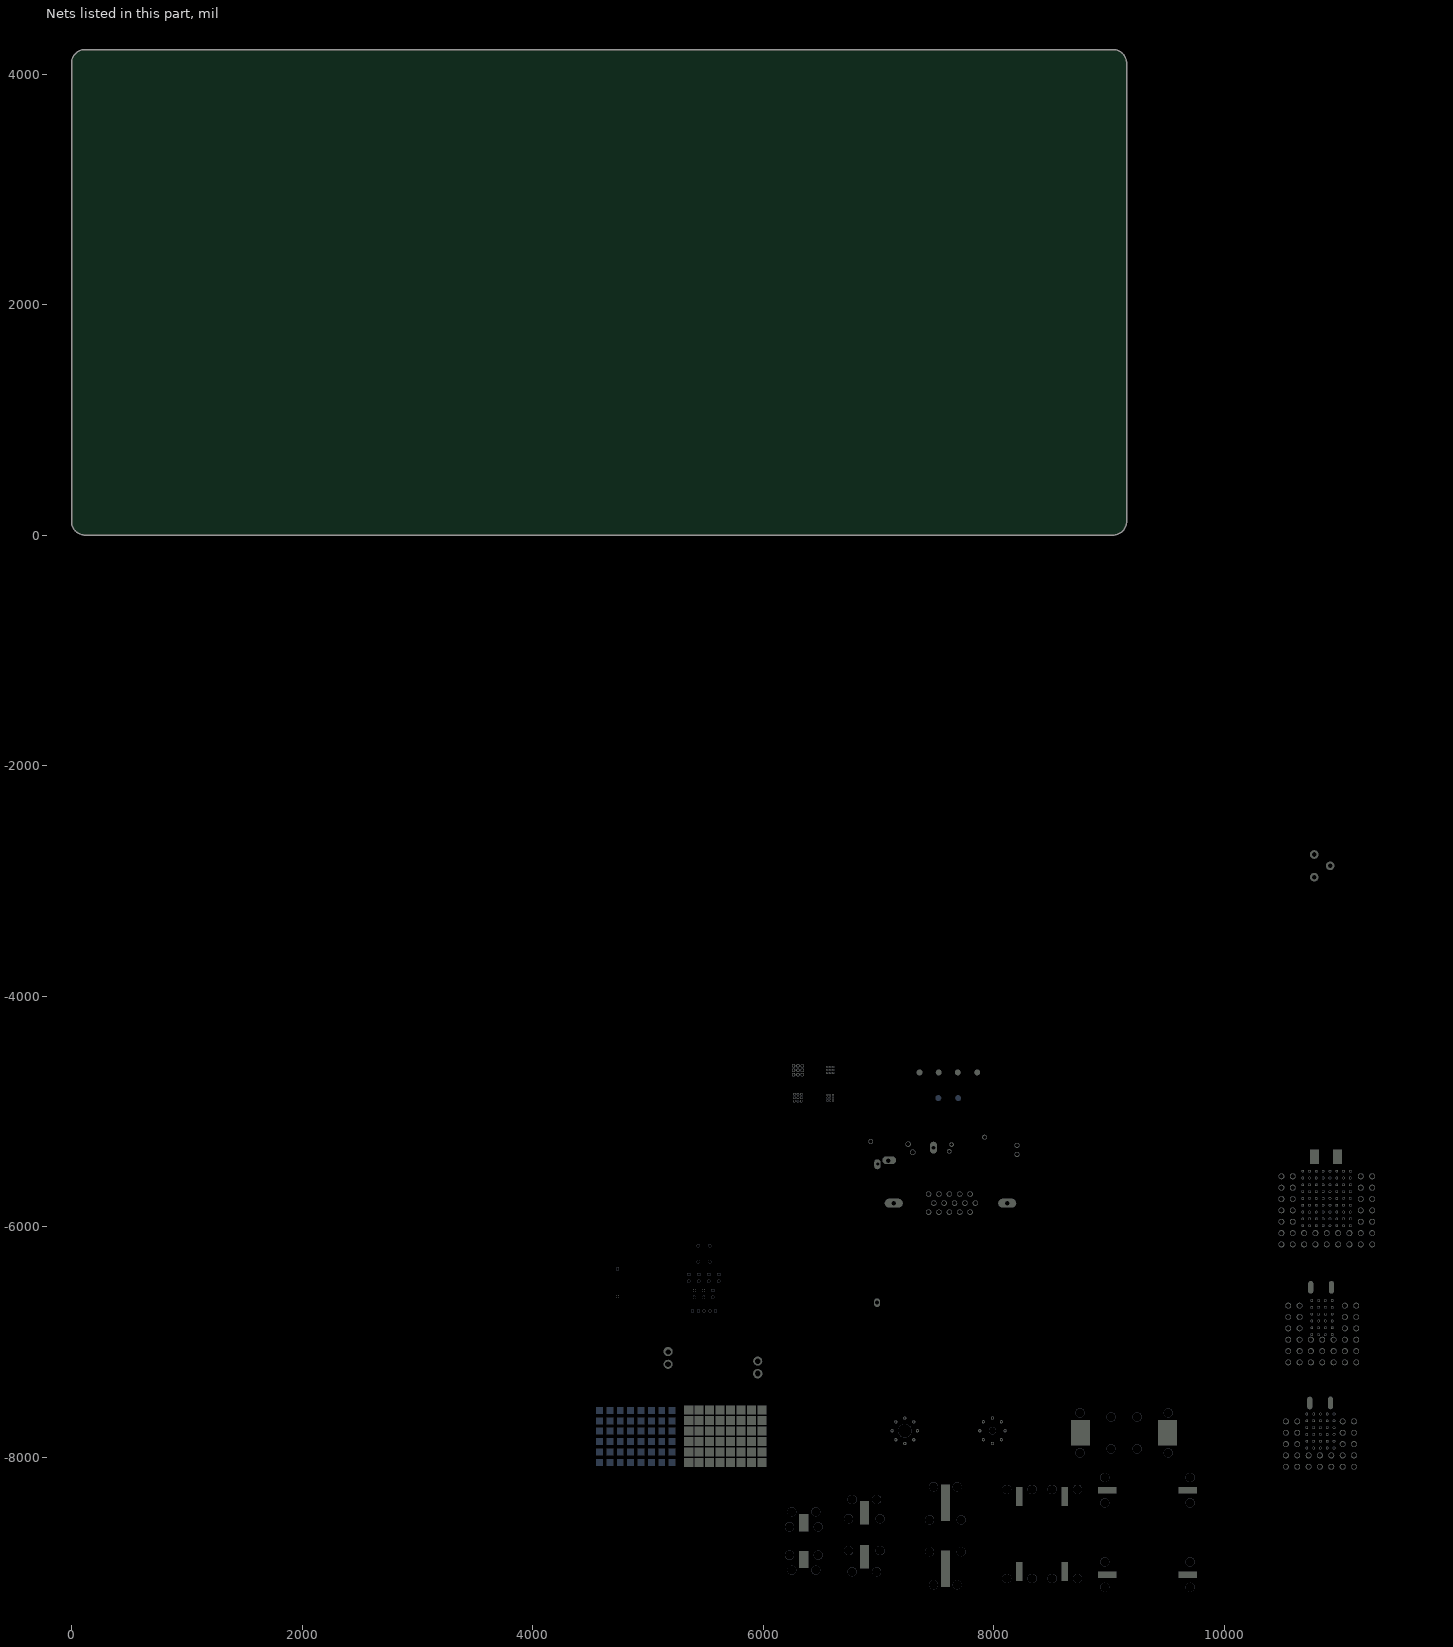
[diagram p0: the nets of this part, all layers, seen from the top]
# Altium PCB MISC86383.PcbDoc (part 2 of 2)
Units mil, origin at the board's own origin, x right, y up, seen from the top; angles counter-clockwise.
Board outline 9153.54 x 4212.6 mil, 2 copper layers (TopLayer, BottomLayer), stack 61.855 mil thick; 21 components, 2 nets, 540 pads, 0 vias.

## Nets (pads, with @x,y where several pads share a name; then routed paths per layer and width w, separated by ;. In a path a pad name is that pad's centre, name@x,y a point inside that pad or via, vN(x,y) a via of type N, cw(c..) or ccw(c..) an arc to the next point about the centre after c; other vN are vias at no path point)
GND: 
RFGND: 
pads on no net: A15XXX.0 AI_V.0 AI_V.1 AI_V.2 M1.0 M2.0 M3.0 M4.0 M5.0 M6.0 MAC.0 Manufacture_Info.0 QR1.0 QR2.0 S/N1.0 S/N2.0 XX.XXXXX.XX.0
copper on no net: | length 3400.6
  TopLayer w5: 966.99,-5983.31 966.99,-5904.57 ; 416.09,-5983.31 1148.12,-5983.31 1148.12,-5904.57 416.09,-5904.57 416.09,-5983.31
  BottomLayer w5: 966.99,-6201.16 966.99,-6122.42 ; 416.09,-6201.16 416.09,-6122.42 1148.12,-6122.42 1148.12,-6201.16 416.09,-6201.16

## Keep-outs
KeepOutLayer:
  rectangle: 416.09,-6580.59 546.29,-6501.85
  lines w5: 966.99,-6580.59 966.99,-6501.85 ; 4541.11,-6803.68 4619.85,-6803.68 ccw(c4619.85,-6685.57) 4737.96,-6685.57 4737.96,-6213.13 ; 4737.96,-6656.59 cw(c4767.4,-6686.21) 4797.02,-6656.78 4797.02,-6803.68 4836.39,-6803.68 ccw(c4836.39,-6685.57) 4954.5,-6685.57 4954.5,-6213.13 ; 4737.96,-6316.89 ccw(c4767.55,-6287.42) 4797.02,-6317.01 4797.02,-6213.13 ; 5281.04,-6265.02 5340.1,-6265.02 5340.1,-6284.67 ccw(c5359.78,-6284.67) 5359.78,-6304.36 5614.11,-6304.36 ccw(c5614.11,-6284.67) 5633.8,-6284.67 5633.8,-6264.99 5692.85,-6265.02 ; 5281.05,-6205.93 5340.1,-6205.93 5340.1,-6186.25 cw(c5359.78,-6186.25) 5359.78,-6166.56 5614.12,-6166.56 cw(c5614.12,-6186.25) 5633.8,-6186.25 5633.8,-6205.93 5692.86,-6205.93 ; 5306.95,-6473.4 ccw(c5277.42,-6443.87) 5306.95,-6414.35 ; 5338.99,-6732.15 ccw(c5309.46,-6702.63) 5338.99,-6673.1 ; 5354.45,-6611.9 ccw(c5324.92,-6582.37) 5354.45,-6552.85 ; 5407.42,-6304.36 ccw(c5338.52,-6235.46) 5407.42,-6166.56 ; 5566.48,-6304.36 cw(c5635.38,-6235.46) 5566.48,-6166.56 ; 5613.5,-6611.9 cw(c5643.03,-6582.37) 5613.5,-6552.85 ; 5637.42,-6732.15 cw(c5666.94,-6702.63) 5637.42,-6673.1 ; 5665.21,-6473.4 cw(c5694.74,-6443.87) 5665.21,-6414.35 ; 0,118.11 ccw(c118.11,118.11) 118.11,0 9035.43,0 ccw(c9035.44,118.11) 9153.55,118.11 9153.55,4094.49 ccw(c9035.44,4094.49) 9035.44,4212.6 118.11,4212.6 ccw(c118.11,4094.49) 0,4094.49 0,118.11 ; 416.09,-6580.59 416.09,-6501.85 1148.12,-6501.85 1148.12,-6580.59 416.09,-6580.59
  lines w47.24: 10850.53,-2998.7 10850.53,-2745.7
  text "KeepOutLayer" at 568.89,-6559.63 h60
  text ".GKO" at 990.7,-6562.54 h60

## Other copper
TopLayer:
  rectangle: 10382.58,-6368.37 11378.64,-5495.37
  rectangle: 10386.51,-7349.73 11311.71,-6621.38
  rectangle: 10441.74,-8196.49 11229.14,-7605.94
  rectangle: 416.09,-5983.31 546.29,-5904.57
  pour cut-out: 8822.66,-7675.58 8822.66,-7903.92 8954.55,-7903.92 8954.55,-7675.58
  pour cut-out: 9440.77,-7675.58 9440.77,-7903.92 9308.88,-7903.92 9308.88,-7675.58
  text "TopLayer" at 582.14,-5960.97 h60
  text ".GTL" at 991.63,-5965.26 h60
BottomLayer:
  rectangle: 416.09,-6201.16 546.29,-6122.42
  region: 7195.27,-5353.48 7195.53,-5353.51 7195.79,-5353.56 7196.04,-5353.62 7196.29,-5353.7 7196.54,-5353.79 7196.77,-5353.9 7197,-5354.03 7197.22,-5354.17 7197.43,-5354.32 7197.63,-5354.49 7197.82,-5354.67 7198,-5354.87 7198.16,-5355.07 7198.31,-5355.28 7198.45,-5355.51 7198.57,-5355.74 7198.67,-5355.98 7198.76,-5356.22 7198.84,-5356.47 7198.89,-5356.73 7198.93,-5356.99 7198.95,-5357.25 7198.96,-5357.51 7198.95,-5357.77 7198.92,-5358.03 7198.87,-5358.29 7198.81,-5358.54 7198.73,-5358.79 7198.64,-5359.03 7198.53,-5359.27 7198.39,-5359.52 7198.38,-5359.54 7148.66,-5442.01 7148.55,-5442.18 7148.53,-5442.21 7148.51,-5442.23 7148.48,-5442.26 7148.24,-5442.51 7147.99,-5442.77 7147.92,-5442.86 7147.83,-5442.94 7147.77,-5443.03 7086.42,-5428.24 7077.67,-5390.77 7077.68,-5390.76 7078.1,-5390.74 7078.11,-5390.74 7078.12,-5390.74 7078.58,-5390.69 7079.04,-5390.63 7079.05,-5390.63 7079.06,-5390.63 7079.52,-5390.54 7079.97,-5390.45 7079.98,-5390.45 7080.42,-5390.32 7080.87,-5390.2 7080.89,-5390.19 7193.51,-5353.74 7193.61,-5353.7 7193.96,-5353.6 7193.97,-5353.6 7194.23,-5353.54 7194.49,-5353.5 7194.75,-5353.48 7195.01,-5353.47
  region: 234 vertices and 0 holes, not listed, extent 6916.92,-5487.07 6998.9,-5378.84
  region: 213 vertices and 0 holes, not listed, extent 7298.33,-5381.42 7368.14,-5337.79
  region: 213 vertices and 0 holes, not listed, extent 7258.39,-5304.82 7332.28,-5264.02
  region: 213 vertices and 0 holes, not listed, extent 6933.97,-5281.24 7007.87,-5240.44
  region: 7666.49,-5323.42 7685.99,-5303.92 7685.99,-5271.01 7689.31,-5267.68 7733.81,-5267.68 7764.31,-5298.18 7764.31,-5336.68 7733.81,-5367.18 7670.31,-5367.18 7666.49,-5363.36
  region: 10094.95,-2791.2 10117.87,-2858.22 10139.56,-2791.2
  region: 10048.25,-2791.2 10071.17,-2858.22 10092.86,-2791.2
  region: 10003.95,-2791.2 10026.87,-2858.22 10048.56,-2791.2
  region: 10140.56,-2962.2 10117.64,-2895.18 10095.95,-2962.2
  region: 10050.56,-2962.2 10027.64,-2895.18 10005.95,-2962.2
  region: 10095.56,-2962.2 10072.64,-2895.18 10050.95,-2962.2
  region: 10303.46,-2795.22 10326.38,-2862.24 10348.07,-2795.22
  region: 10346.77,-2795.22 10369.69,-2862.24 10391.38,-2795.22
  region: 10258.64,-2795.2 10281.56,-2862.22 10303.25,-2795.2
  region: 10304.25,-2961.2 10281.33,-2894.18 10259.64,-2961.2
  region: 10349.56,-2961.2 10326.64,-2894.18 10304.95,-2961.2
  region: 10394.56,-2961.2 10371.64,-2894.18 10349.95,-2961.2
  region: 10040.56,-2670.7 10017.64,-2603.68 9995.95,-2670.7
  region: 9992.77,-2499.72 10015.69,-2566.74 10037.38,-2499.72
  region: 10472.56,-2669.7 10449.64,-2602.68 10427.95,-2669.7
  region: 10425.95,-2503.7 10448.87,-2570.72 10470.56,-2503.7
  region: 10707.5,-2500.19 10730.42,-2567.21 10752.11,-2500.19
  region: 10663.89,-2500.19 10686.81,-2567.21 10708.5,-2500.19
  region: 10576.27,-2500.19 10599.2,-2567.21 10620.89,-2500.19
  region: 10620.27,-2500.19 10643.2,-2567.21 10664.89,-2500.19
  region: 10709.34,-2669.66 10686.42,-2602.65 10664.73,-2669.66
  region: 10753.34,-2669.66 10730.42,-2602.65 10708.73,-2669.66
  region: 10665.73,-2669.66 10642.81,-2602.65 10621.12,-2669.66
  region: 10622.12,-2669.66 10599.2,-2602.65 10577.51,-2669.66
  region: 10428.56,-2669.7 10405.64,-2602.68 10383.95,-2669.7
  region: 10383.56,-2669.7 10360.64,-2602.68 10338.95,-2669.7
  region: 10338.25,-2669.7 10315.33,-2602.68 10293.64,-2669.7
  region: 10292.64,-2503.7 10315.56,-2570.72 10337.25,-2503.7
  region: 10380.77,-2503.72 10403.69,-2570.74 10425.38,-2503.72
  region: 10337.46,-2503.72 10360.38,-2570.74 10382.07,-2503.72
  region: 10129.56,-2670.7 10106.64,-2603.68 10084.95,-2670.7
  region: 10084.56,-2670.7 10061.64,-2603.68 10039.95,-2670.7
  region: 10174.56,-2670.7 10151.64,-2603.68 10129.95,-2670.7
  region: 10037.95,-2499.7 10060.87,-2566.72 10082.56,-2499.7
  region: 10082.25,-2499.7 10105.17,-2566.72 10126.86,-2499.7
  region: 10128.95,-2499.7 10151.87,-2566.72 10173.56,-2499.7
  text ".GBL" at 991.31,-6179.49 h60
  text "BottomLayer" at 568.89,-6180.99 h60

## Silkscreen, mask and mechanical layers (free items; w line width, h text height)
TopOverlay:
  drawing of 754 lines, arcs and shapes, not listed
  text "Solder Mask:" at 281.2,-1022.86 h60
  text "IPC SM-840" at 693.7,-1023.86 h60
  text "Silkscreen Color:" at 1459.7,-1023.86 h60
  text "White" at 1938.7,-1023.86 h60
  text "Units:" at 1459.7,-1122.86 h60
  text "PTH Copper Thickness:" at 281.2,-1123.86 h60
  text ">20um" at 954.7,-1124.86 h60
  text "mm" at 1657.7,-1124.36 h60
  text "Dielectric Constant Er@1GHz To 1MHz:" at 280.87,-1222.83 h60
  text "4.2 --- 4.6" at 1460.37,-1222.33 h60
  text "Panel Size:" at 279.2,-1321.36 h60
  text "2L,n,000.00×000.00mm,FR4(TG130/170-CTI175/600),1/2OZ,Green/Blue,OSP/HAL_LF,1.6/1.2/1.0/0.8mm" at 584.37,-1321.33 h60
  text "Silkscreen on PTH:" at 279.7,-1422.86 h60
  text "Primary Side Retained;" at 797.7,-1423.86 h60
  text "Secondary Side  Removed for Soldering" at 1459.7,-1425.36 h60
  text "Special Requirements" at 278.69,-1513.54 h60
  text "工程问题2小时内没回复，请电联" at 2165.37,-1520.83 h60
  text "1. Lead-free HASL (HAL_LF, Lead Free Hot Air Leveling)" at 869.58,-1617.13 h60
  text "2. Organic Solderability Preservative (OSP, Organic Solderability Preservatives)" at 869.58,-1701.13 h60
  text "Dolby silkscreen" at 4512.37,-1708.95 h60
  text "Dolby certification silkscreen" at 6112.87,-1708.95 h60
  text "Reserved boundary for support chain" at 8462.87,-1708.95 h60
  text "3. Electroless Nickel Immersion Gold (ENIG, Electroless Nickel/Immersion Gold)" at 868.08,-1792.63 h60
  text "Plated Technics" at 353.7,-1827.36 h60
  text "Character spec: font Arial (TrueType) bold, character height 100mil" at 6259.87,-1832.83 h80
  text "Double-D silkscreen graphic must not be placed on holes ≥0.5mm" at 4568.87,-1844.83 h60
  text "4. ENIG + gold finger (ENIG_G/F, Electroless Nickel/Immersion Gold + Gold Finger)" at 869.58,-1873.13 h60
  text "Keep-out area, same side: no other logos, marks, graphics, text silkscreen or exposed copper" at 4568.37,-1917.33 h60
  text "5. Gold plating (Gold_plated, Gold-plated)" at 870.58,-1953.63 h60
  text "6. Gold plating + gold finger (Gold_Plated_G/F, Gold-plated + Gold Finger)" at 871.08,-2031.63 h60
  text "Bottom silkscreen layer" at 7066.37,-2212.83 h80
  text "35.0mm*5.4mm" at 6267.37,-2223.33 h80
  text "Impedance Control" at 283.44,-2260.22 h60
  text "Target Impedance" at 1080.27,-2260.12 h60
  text "Layer(s)" at 2594.41,-2260.04 h60
  text "Width & Clearance" at 1826.1,-2260.35 h60
  text "Fabrication mark" at 6112.87,-2351.83 h60
  text "Barcode frame" at 6862.37,-2351.83 h60
  text "Panel separation V-CUT" at 8468.5,-2353 h60
  text "Power section: content to be added" at 10159.08,-2354.63 h196.85
  text "75 +/- 10% Ohm" at 1092.97,-2366.32 h60
  text "G/12/14.5/12/G mil" at 1774.02,-2367 h60
  text "layer 1" at 2584.91,-2366.88 h60
  text "Single End Impedance" at 283.44,-2407.04 h60
  text "75 +/- 10% Ohm" at 1092.97,-2464.32 h60
  text "G/7/6.9/7/G mil" at 1774.02,-2465 h60
  text "layer 1" at 2584.91,-2464.88 h60
  text "Do not place on differential pair or DDR signal lines" at 7141.37,-2531.33 h80
  text "[ Zo ]" at 506.94,-2544.29 h60
  text "V-CUT top blade diagram" at 8949.31,-2561.75 h60
  text "50 +/- 10% Ohm" at 1091.02,-2563.5 h60
  text "layer 1" at 2583.52,-2565 h60
  text "G/5/22/5/G mil" at 1774.02,-2567 h60
  text "HOT" at 11123,-2637.31 h196.85
  text "20mm" at 9161.31,-2658.42 h30
  text "G/5/6.1/5/6.1/5/G mil" at 1784.02,-2758 h60
  text "100 +/- 10% Ohm" at 1079.97,-2759.01 h60
  text "layer 1" at 2595.9,-2760.79 h60
  text "Differential Impedance" at 283.3,-2808.62 h60
  text "15mm" at 9158.31,-2811.9 h30
  text "7.2/4/7.2 mil" at 1782.07,-2857.18 h60
  text "100 +/- 10% Ohm" at 1078.02,-2858.19 h60
  text "layer 1" at 2593.95,-2859.97 h60
  text "COLD" at 11094.26,-2876.56 h196.85
  text "[ Zo ]" at 506.43,-2931.95 h60
  text "100 +/- 10% Ohm" at 1077.97,-2959.51 h60
  text "G/4/13/4/24/4/13/4/G mil" at 1785.02,-2961 h60
  text "layer 1" at 2593.9,-2961.29 h60
  text "10mm" at 9157.31,-3008.75 h30
  text "( G: Ground )" at 416.51,-3039.45 h60
  text "90 +/- 10% Ohm" at 1106.02,-3057 h60
  text "layer 1" at 2591.9,-3057.79 h60
  text "G/5/9.2/5/9.2/5/G mil" at 1784.02,-3060.5 h60
  text "F" at 11306.54,-3110.41 h157.48
  text "T3.15AL 250V~" at 10456.37,-3139.22 h78.74
  text "5mm" at 9155.31,-3205.75 h30
  text "layer 1" at 2594.02,-3251 h60
  text "30 +/- 10% Ohm" at 1101.08,-3256.13 h60
  text "G/4/13/4/24/4/13/4/G mil" at 1785.52,-3258.5 h60
  text "Common Mode Impedance" at 263.08,-3261.13 h60
  text "2.5mm" at 9154.31,-3302.75 h30
  text "T3.15AH 250V~" at 10459.37,-3340.72 h78.74
  text "[ Zc ]" at 511.08,-3342.13 h60
  text "T5AH 250V~" at 10473.37,-3538.72 h78.74
  text "1" at 6212.28,-3542.13 h160
  text "2" at 6338.78,-3542.13 h160
  text "3" at 6489.49,-3541.68 h160
  text "4" at 6635.21,-3542.38 h160
  text "Refer to Gerber documents GTP&GBP for Stencil aperture design" at 1178.13,-3606.32 h60
  text "[X, X-compatible SMD parts (FFC, chips, modules, ...) pads with separate stencil openings]" at 1177.41,-3693.74 h60
  text "Stencil (Stencil)" at 277.37,-3703.33 h60
  text "CAUTION:" at 10092.37,-3744.22 h51.18
  text "Process direction" at 4512.37,-3756.95 h60
  text "Screw position mark" at 6112.37,-3756.95 h60
  text "Board model" at 6862.37,-3757.45 h60
  text "FOR CONTINUED PROTECTION" at 10092.37,-3799.34 h59.06
  text "New / The same as X.XXXX / Refer to<X.XXXX Stencil Revision Explanation>" at 1176.03,-3800.88 h60
  text "AGAINST RISK OF FIRE REPLACE" at 10084.49,-3846.58 h59.06
  text "ONLY WITH SAME TYPE AND" at 10064.81,-3897.76 h59.06
  text "Test fixture (Testing jig)" at 275.46,-3898.98 h60
  text "New / The same as X.XXXX / Refer to<X.XXXX Testing jig Revision Explanation>" at 1177.24,-3899.94 h60
  text "[ No Need ]" at 3417.51,-3902.93 h60
  text "RATING OF FUSE" at 10084.49,-3952.88 h59.06
  text "Wave-soldering fixture (Wave-soldering jig)" at 277.67,-3997.22 h60
  text "New / The same as X.XXXX / Refer to<X.XXXX Wave-soldering jig Revision Explanation>" at 1178.1,-3997.09 h60
  text "LED+" at 11211.53,-4003.8 h48.31 r90
  text "LED-" at 11252.33,-4004 h48.31 r90
  text "LED DRIVER" at 10573.37,-4095.22 h60
  text "Solder paste/Red plastic" at 1175.65,-4099 h60
  text "Production process" at 276.15,-4100.5 h60
  text "12V" at 11204.43,-4136.2 h50 r90
  text "GND" at 11256.87,-4150.72 h50 r90
  text "[Process and notes]" at 456.37,-4185.33 h60
  text "AC IN" at 10573.37,-4210.22 h60
  text "DC IN" at 10578.37,-4295.22 h60
  text "Special requirements (Special Requirements)" at 277.15,-4298.5 h60
  text "DC OUT" at 10578.37,-4380.22 h60
  text "SMD parts over 2mm high on wave-solder side" at 276.87,-4399.83 h60
  text "Dummy via" at 6112.37,-4422.45 h60
  text "MARK" at 6862.37,-4422.45 h60
  text "Board size limit" at 8462.37,-4422.45 h60
  text "INVERTER" at 10580.37,-4453.22 h60
  text "Packaging notes (Package Attention)" at 276.53,-4496.05 h60
  text "6.2mil" at 6376.87,-4525.83 h60
  text "PWR UPGRADE" at 10534.61,-4529.97 h60
  text "Recommended value" at 8923.53,-4540.65 h80
  text "Limit value" at 9414.46,-4540.92 h80
  text "[Easily damaged components]" at 517.87,-4580.83 h60
  text ">100X100mm" at 8984.37,-4608.83 h50
  text "<330X250mm" at 8983.87,-4650.83 h50
  text "T1.2mm" at 8801.87,-4651.33 h50
  text "<400X330mm" at 9382,-4653.5 h50
  text "SMT" at 8509.5,-4666.5 h80
  text "T1.6mm" at 8802.37,-4693.83 h50
  text "<350X300mm" at 8984.87,-4693.33 h50
  text "New footprint matching (Footprint Matching)" at 276.53,-4696.05 h60
  text "<330X250mm" at 8890,-4758.5 h50
  text "<345X310mm" at 9382,-4758.5 h50
  text "AI" at 8509.5,-4772.5 h80
  text "0.8/0.5mm" at 6182.37,-4774.33 h60
  text "0.5/0.3mm" at 6461.37,-4774.33 h60
  text "[New component footprint]" at 503.87,-4779.83 h60
  text "W<220mm" at 8920.08,-4851.5 h50
  text "W<260mm" at 9411.58,-4851.5 h50
  text "Wave soldering" at 8509.5,-4865 h80
  text "(Automated Testing Support)" at 594.87,-4894.33 h45
  text "Automatic test support" at 276.37,-4897.83 h60
  text "<340X290mm" at 8890,-4945.5 h50
  text "<400X300mm" at 9382,-4945.5 h50
  text "CNC depaneling" at 8483,-4955 h80
  text "[Reserved suction cup and press pin positions]" at 436.87,-4982.33 h60
  text "0.6/0.4mm" at 6182.37,-5015.83 h60
  text "0.45/0.25mm" at 6462.37,-5015.33 h60
  text "Isolation barrier" at 10708.93,-5121.7 h78.74
  text "Automatic test" at 4512.37,-5136.45 h60
  text "Safety-approval silkscreen" at 6112.37,-5136.45 h60
  text "Drag-solder pad" at 6862.37,-5136.45 h60
  text "Support post" at 8462.37,-5136.45 h60
  text "2.0mm" at 7034.87,-5276.33 h60
  text "Layer Stack Up Detail for" at 417.47,-5341.86 h100
  text ".Pcb_File_Name_No_Path" at 1478.29,-5341.86 h100
  text "48W (32 inch) board, primary flyback SMD MOS top/bottom copper heat area >550 mm2" at 11136.95,-5384.23 h60
  text "!" at 6267.85,-5401.91 h180
  text "!" at 6646.16,-5405.01 h180
  text "40W/48W/65W/75W/108W board, 12V SMD rectifier top/bottom copper heat area >550 mm2" at 11136.95,-5443.28 h60
  text "F3.15AL/250V" at 6147.77,-5485.29 h50
  text "F3.15AL/32V" at 6531.18,-5485.51 h50
  text "RJ45" at 7293.37,-5487.83 h60
  text "DIP" at 8249.87,-5488.33 h60
  text "Layer" at 581.83,-5489.59 h50
  text "Gerber" at 953.54,-5489.59 h50
  text "Layer" at 1264.69,-5489.59 h50
  text "Layer" at 1900.93,-5489.59 h50
  text "Copper" at 2689.83,-5489.59 h50
  text "Dielectric" at 3001.61,-5489.59 h50
  text "USB3" at 7619.87,-5490.33 h60
  text "DIP" at 7959.87,-5490.83 h60
  text "Stack up" at 1900.93,-5540.47 h50
  text "Height" at 3001.61,-5540.47 h50
  text "Name" at 581.83,-5541.97 h50
  text "Document" at 953.54,-5541.97 h50
  text "Ordor" at 1264.69,-5541.97 h50
  text "Thickness" at 2689.83,-5541.97 h50
  text "HEADPHONE" at 6895.91,-5556.24 h60
  text "25mm*22mm" at 11441.67,-5583.08 h60
  text "Wire clip" at 6112.37,-5632.95 h60
  text "TopOverlay" at 581.53,-5774.82 h60
  text ".GTO" at 991.1,-5777.38 h60
  text "Top-layer support post" at 8549.5,-5810 h60
  text "Ø8mm, Ø10mm" at 5437.37,-5829.33 h60
  text "Ø10mm, Ø12mm" at 4691.37,-5830.83 h60
  text "0.4mil" at 2998.93,-5862.41 h60
  text "Corresponding press pin diameter:" at 5439.37,-5916.83 h60
  text "Corresponding suction cup diameter:" at 4693.37,-5918.33 h60
  text "1" at 1317.89,-5965.56 h60
  text "1.4mil" at 2702.89,-5965.62 h60
  text "Pointed Ø4mm, flat Ø6mm" at 5437.37,-6002.83 h60
  text "Ø8mm, Ø10mm" at 4691.37,-6004.33 h60
  text "Stamp holes & process rail" at 4512.37,-6140.45 h60
  text "Reserved" at 6112.37,-6140.45 h60
  text "Conductive foam" at 6862.37,-6140.45 h60
  text "AI fixture" at 8462.37,-6140.45 h60
  text "2" at 1317.95,-6178.6 h60
  text "1.4mil" at 2701.18,-6179.61 h60
  text "TUNER" at 5720.87,-6257.83 h60
  text "0.4mil" at 3001.6,-6274.29 h60
  text "75W (<42 inch) board, constant-current SMD MOS top/bottom copper heat area >420 mm2" at 11136.93,-6556.7 h60
  text "1.5mm" at 5726.87,-6595.33 h60
  text "23.5mm*18.5mm" at 11365.43,-6725.2 h60
  text "Board thickness 1.2mm, non-rail side ≤270mm: V-cut connection" at 4978.37,-6817.83 h60
  text "HDMI" at 7204.42,-6821.03 h78.74
  text "TUNER" at 7845.87,-6821.83 h78.74
  text "Board thickness 1.6mm, non-rail side ≤320mm: V-cut connection" at 4977.87,-6897.33 h60
  text "AI (1.5+4mm)" at 4596.87,-6900.83 h60
  text "Keep-out area, bottom layer: no components; no non-ground net pins or component pads" at 6873.87,-6919.83 h78.74
  text "White solder mask ink" at 4512.37,-7016.95 h60
  text "Process related" at 6112.37,-7016.95 h60
  text "Cable routing" at 6862.37,-7016.95 h60
  text "QR code" at 8469.87,-7020.83 h78.74
  text "Routed slot boundary" at 6197.04,-7221.63 h60
  text "BoardCutout" at 6154.12,-7289.46 h60
  text "D 2.0mm" at 6572.87,-7312.83 h60
  text "LVDS Cable (7mm)" at 7407.37,-7409.83 h60
  text "SCART||AV" at 5842.87,-7412.83 h50
  text "SCART (right-angle connector)||AV" at 5008.37,-7414.83 h50
  text "Tinned pad" at 4512.37,-7510.45 h60
  text "Fabrication V-CUT" at 6112.37,-7510.45 h60
  text "Locating hole" at 6862.37,-7510.45 h60
  text "FUSE(T5AH 250V~)-S" at 8871.37,-7537.83 h60
  text "40W/48W (<32 inch) board, secondary constant-current SMD MOS top/bottom copper heat area >300 mm2" at 11132.93,-7563.2 h60
  text "Fabricator: new V-CUT blade" at 6229.37,-7702.33 h60
  text "20mm*15mm" at 11353.43,-7759.2 h60
  text "2.0mm" at 6517.75,-7827.38 h20
  text "45°" at 6494.95,-7895.99 h20
  text "2.4mm" at 6334.45,-7906.99 h20
  text "BGA Room" at 4512.37,-8170.94 h60
  text "Through-hole reflow hole" at 6112.37,-8170.94 h60
  text "L/LC4/19.6*21.8-S-1" at 9119.87,-8171.33 h60
  text "L/LC2/RM06*4-VS" at 8207.37,-8183.83 h60
  text "EC(18*16.5)-S" at 7419.37,-8190.83 h60
  text "EC(10*10.5)-S" at 6200.37,-8277.83 h60
  text "EC(12.5*14)-S" at 6741.37,-8278.33 h60
  text "EC(10*12.4)-S" at 6201.87,-8336.83 h60
  text "0.65 pitch" at 5182.87,-8483.33 h60
  text "0.65pitch的BGA芯片＞2颗，需增加规则" at 4840.37,-8654.83 h60
BottomOverlay:
  drawing of 73 lines, arcs and shapes, not listed
  text "HOT" at 11496.32,-2642.44 h196.85
  text "COLD" at 11577.77,-2875.44 h196.85
  text "2.5mm" at 9153.37,-3627.33 h25
  text "5mm" at 9156.31,-3715.75 h30
  text "NC" at 11322.23,-3737.52 h51.18 r270
  text "+" at 11305.93,-3744.7 h78.74
  text "-" at 11399.93,-3750.7 h118.11
  text "10mm" at 9162.31,-3916.75 h30
  text "FB1" at 11333.33,-3985 h48.31 r270
  text "14m" at 9160.31,-4031.75 h30
  text "LED DRIVER" at 10468.37,-4095.22 h60
  text "V-CUT bottom blade diagram" at 8948.31,-4128.75 h60
  text "AC IN" at 10468.37,-4210.22 h60
  text "DC IN" at 10468.37,-4295.22 h60
  text "DC OUT" at 10468.37,-4380.22 h60
  text "INVERTER" at 10467.37,-4451.22 h60
  text "PWR UPGRADE" at 10467.37,-4531.22 h60
  text ".GBO" at 991.72,-6369.9 h60
  text "BottomOverlay" at 570.05,-6370.89 h60
TopPaste:
  drawing of 278 lines, arcs and shapes, not listed
  text "TopPaste" at 581.53,-5678.29 h60
  text ".GTP" at 991.1,-5680.42 h60
BottomPaste:
  rectangle: 416.09,-6487.08 546.29,-6408.34
  lines w5: 966.99,-6487.08 966.99,-6408.34 ; 416.09,-6487.08 416.09,-6408.34 1148.12,-6408.34 1148.12,-6487.08 416.09,-6487.08
  text "BottomPaste" at 568.89,-6464.1 h60
  text ".GBP" at 991.99,-6469.22 h60
TopSolder:
  drawing of 278 lines, arcs and shapes, not listed
  text "TopSolder" at 582.03,-5869.37 h60
  text ".GTS" at 991.1,-5871.02 h60
BottomSolder:
  drawing of 48 lines, arcs and shapes, not listed
  text "BottomSolder" at 568.89,-6277.69 h60
  text ".GBS" at 991.07,-6278.58 h60
3D和装配:
  circle w5: c7989.37,-7770.83 r354.33
  circle w4: c7989.37,-7770.83 r236.22
  circle w4: c7229.37,-7771.33 r137.8
  lines w5: 0,118.11 0,0 118.11,0 ; 7008.29,-6730.39 7539.78,-6730.39 7539.78,-6198.89 7008.29,-6198.89 7008.29,-6730.39 ; 7692.18,-6730.39 8223.68,-6730.39 8223.68,-6198.89 7692.18,-6198.89 7692.18,-6730.39
自动测试:
  circle w6: c4901.52,-5495.83 r196.85
  circle w6: c4902.65,-5495.83 r236.22
  circle w3: c5656.52,-5492.33 r196.85
  circle w3: c5657.65,-5492.33 r236.22
端子视图:
  circle w1.97: c7989.37,-7770.83 r49.21
  circle w1.97: c7989.37,-7770.83 r39.37
  circle w1.97: c7989.37,-7770.83 r31.5
  circle w1.97: c7989.37,-7770.83 r98.43
  circle w1.97: c7989.37,-7770.83 r64.96
  circle w1.97: c7989.37,-7770.83 r68.9
  circle w1.97: c7989.37,-7770.83 r78.74
  circle w1.97: c7989.37,-7770.83 r88.58
  circle w1.97: c7989.37,-7770.83 r59.06
  circle w1.97: c7229.37,-7771.33 r59.06
  lines w275.59: 7332.05,-7209.84 7930.47,-7209.84
顶层限制:
  circle w5: c6463.47,-5871.84 r137.8
底层限制:
  circle w5: c6463.47,-5871.84 r98.43
附加说明:
  region: 5637.42,-6673.1 5637.42,-6732.15 5338.99,-6732.15 5338.99,-6673.1 hole: 5477,-6702.63 5488.2,-6691.43 5499.4,-6702.63 5488.2,-6713.83
  region: 5613.5,-6552.85 5613.5,-6611.9 5354.45,-6611.9 5354.45,-6552.85 hole: 5472.77,-6582.37 5483.97,-6571.17 5495.17,-6582.37 5483.97,-6593.57
  region: 5306.95,-6473.4 5306.95,-6414.35 5665.21,-6414.35 5665.21,-6473.4 hole: 5474.88,-6443.87 5486.08,-6432.67 5497.28,-6443.87 5486.08,-6455.07
  region: 5614.12,-6166.56 5614.11,-6304.36 5359.78,-6304.36 5359.78,-6166.56 hole: 5475.75,-6235.46 5486.95,-6224.26 5498.15,-6235.46 5486.95,-6246.66
  lines w5: 4489.03,-1489.01 5619.03,-1489.01 ; 4489.03,-1381.68 5619.03,-1381.68 ; 4489.03,-1274.35 5619.03,-1274.35 ; 4489.03,-1167.01 5619.03,-1167.01 ; 4489.03,-1059.68 5919.53,-1059.68 ; 4789.53,-1596.35 4789.53,-952.35 ; 5619.03,-1596.35 5619.03,-952.35 ; 5972.53,-1489.01 7941.03,-1489.01 ; 5972.53,-1381.68 7941.03,-1381.68 ; 5972.53,-1274.35 7941.03,-1274.35 ; 5972.53,-1167.01 7941.03,-1167.01 ; 5972.53,-1059.68 7941.03,-1059.68 ; 6077.03,-1596.35 6077.03,-1059.68 ; 4489.03,-1596.35 4489.03,-952.35 5919.53,-952.35 5919.53,-1596.35 4489.03,-1596.35 ; 5972.53,-1596.35 7941.03,-1596.35 7941.03,-952.35 5972.53,-952.35 5972.53,-1596.35
  text "Keep the description brief so derived projects or board revisions can inherit it:" at 6376.87,-997.33 h35
  text "Template date:" at 2292.87,-1024.33 h60
  text "Version cycle number" at 4510.87,-1025.5 h60
  text "PCB designer" at 5066.37,-1026 h60
  text "Customer" at 5729.37,-1025.5 h60
  text "Special notes" at 6003.87,-1025.5 h60
  text "2019.12.06" at 2614.87,-1027.83 h60
  text "For new or special design rules: hole spacing for the Bangladesh region; special safety clearance; special stackup not allowed to change; support chain; designated factory..." at 6376.37,-1042.83 h35
  text "Material utilization:" at 2292.37,-1121.33 h60
  text "8X%" at 2614.87,-1125.33 h60
  text "(Fill in for non-TV division projects)" at 2804.87,-1125.33 h60
  text "A19XXX" at 4530.37,-1132.5 h60
  text "1" at 6013.87,-1132.5 h60
  text "XXXXXXXX" at 4834.37,-1133.33 h60
  text "2" at 6013.82,-1239.66 h60
  text "XXXXXX" at 5658.37,-1342.83 h60
  text "3" at 6013.87,-1346.66 h60
  text "4" at 6013.87,-1454.66 h60
  text "① Panel production, single-board shipment" at 1726.87,-1489.33 h30
  text "Fabrication special requirements; leave blank if none;" at 883.03,-1521.99 h60
  text "Reference:" at 1591.87,-1522.83 h60
  text "② 4-up panel production, 2-up panel shipment" at 1726.37,-1533.33 h30
  text "5" at 6013.87,-1561.66 h60
  text "Copy the notes below to the TopOverlay layer; one or two items may be noted" at 1880.37,-4102.83 h60
  text "Only one barcode position on board; the other barcode goes on a component" at 3399,-4105.73 h60
  text "SMD parts 3.5mm from PCB rail edge; production needs special control" at 1175.37,-4184.83 h60
  text "No barcode position on board; barcode goes on a component" at 3399,-4184.93 h60
  text "Customer special requirements; special process requirements; leave blank if none" at 1173.42,-4297.79 h60
  text "Height and designators of SMD parts over 2mm on solder side; leave blank if none" at 1173.42,-4397.79 h60
  text "Easily damaged component designators; leave blank if none" at 1171.65,-4543.95 h60
  text "New footprint designators; leave blank if none" at 1174.02,-4751 h60
  text "Suction cup and press pin positions reserved: enter \"Yes\", otherwise \"No\"" at 1174.87,-4953.83 h60
  text "X.XXXX.XXX Stencil Revision Explanation" at 250.62,-6864.92 h60
  text "X.XXXX.XXX Testing jig Revision Explanation" at 250.12,-6933.92 h60
  text "X.XXXX.XXX Wave-soldering jig Revision Explanation" at 249.62,-7001.92 h60
DrillDrawing:
  text ".Legend" at 255.69,-904.11 h60